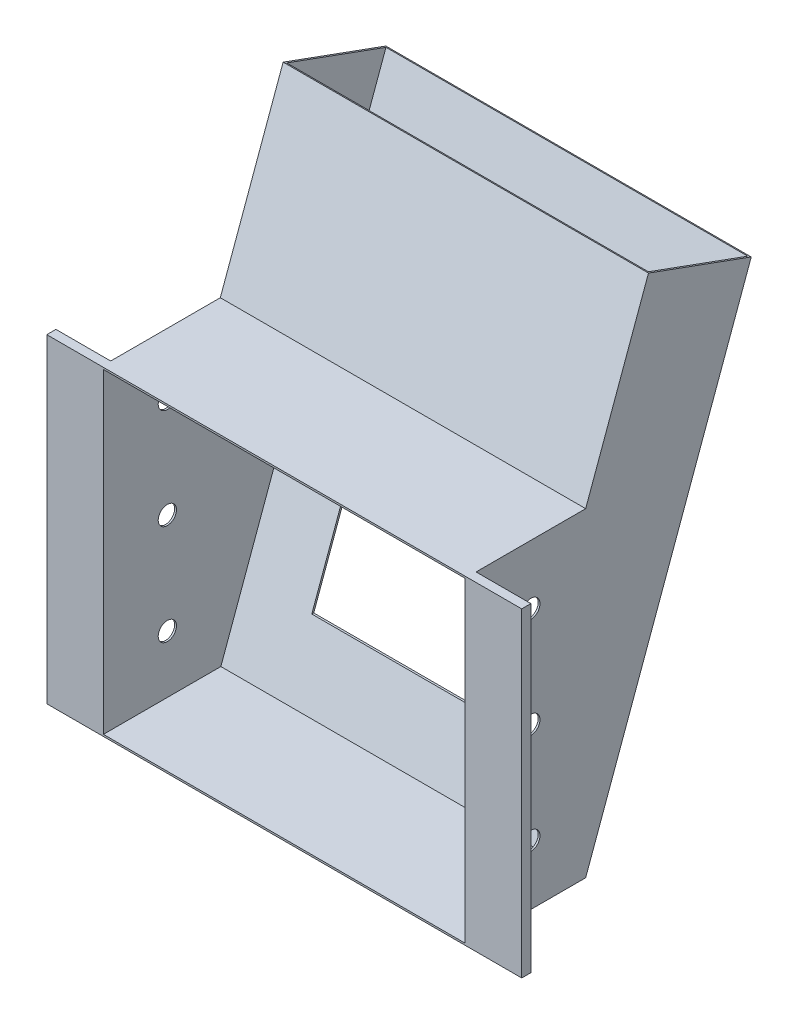
from build123d import *

# Parameters (mm, degrees)
SKETCH_1_W          = 400
SKETCH_1_H          = 350
EXTRUDE_1_DEPTH     = 130
EXTRUDE_5_DEPTH     = 400
SHELL_2_T           = -2
SKETCH_3_W          = 60
SKETCH_3_H          = 350
EXTRUDE_2_DEPTH     = 10
SKETCH_8_W          = 250
SKETCH_8_H          = 200
CUT_EXTRUDE_1_DEPTH = 545.949881083
SKETCH_9_R          = 10
CUT_EXTRUDE_2_DEPTH = 614.954393374


with BuildPart() as part:
    # 草图1 → 凸台-拉伸1 (new body)
    with BuildSketch(Plane.XY):
        Rectangle(SKETCH_1_W, SKETCH_1_H)
    extrude(amount=EXTRUDE_1_DEPTH)

    # 草图7 → 凸台-拉伸5 (add)
    with BuildSketch(Plane.ZY.offset(200)):
        Polygon((0, 175), (-68.782844267, 363.979311471), (-181.270675963, 323.037089017), (0, -175), align=None)
    extrude(amount=-EXTRUDE_5_DEPTH)

    # 抽壳2
    shell_2_openings = [part.faces().sort_by_distance(p)[0] for p in [
        (0, 0, 130),
        (0, 343.508200244, -125.026760115),
    ]]
    offset(amount=SHELL_2_T, openings=shell_2_openings, kind=Kind.INTERSECTION)

    # 草图3 → 凸台-拉伸2 (add)
    with BuildSketch(Plane.XY.offset(130)):
        with Locations((-230, 0)):
            Rectangle(SKETCH_3_W, SKETCH_3_H)
        with Locations((230, 0)):
            Rectangle(SKETCH_3_W, SKETCH_3_H)
    extrude(amount=-EXTRUDE_2_DEPTH)

    # 草图8 → 切除-拉伸1 (cut, through all)
    with BuildSketch(Plane.XY.offset(130)):
        Rectangle(SKETCH_8_W, SKETCH_8_H)
    extrude(amount=-CUT_EXTRUDE_1_DEPTH, mode=Mode.SUBTRACT)

    # 草图9 → 切除-拉伸2 (cut, through all)
    with BuildSketch(Plane(origin=(200, 0, 0), x_dir=(0, 0, -1), z_dir=(1, 0, 0))):
        with Locations((-60, 110)):
            Circle(SKETCH_9_R)
        with Locations((-60, -110)):
            Circle(SKETCH_9_R)
        with Locations((-60, 0)):
            Circle(SKETCH_9_R)
    extrude(amount=-CUT_EXTRUDE_2_DEPTH, mode=Mode.SUBTRACT)


solid = part.part
